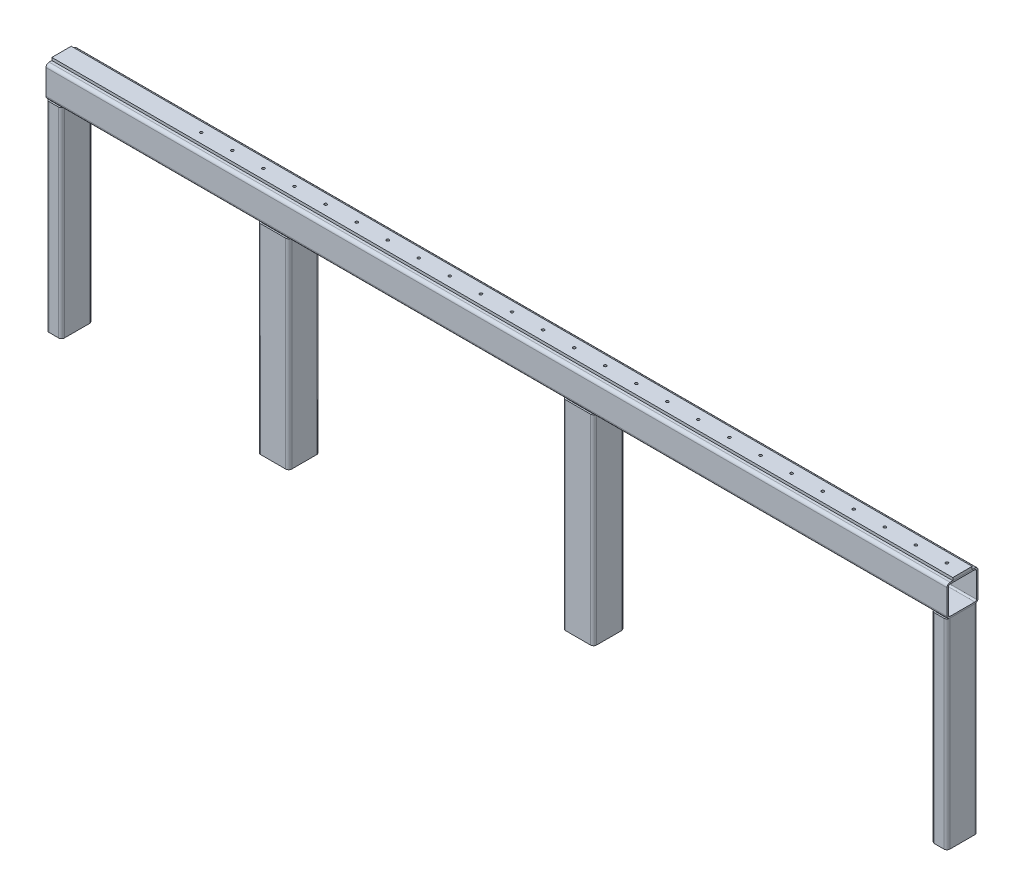
SolidWorks part; units mm, degrees
material "Q235"
ref_plane "Front Plane" through (0, 0, 0) normal (0, 0, 1) x (1, 0, 0)
ref_plane "Top Plane" through (0, 0, 0) normal (0, 1, 0) x (1, 0, 0)
ref_plane "Right Plane" through (0, 0, 0) normal (1, 0, 0) x (0, 0, -1)
sketch "草图1" plane through (0, 0, 0) normal (0, 0, 1) x (1, 0, 0)
  line L0 (0, 0) -> (0, 515)
  line L1 (0, 515) -> (2280, 515)
  line L2 (2280, 515) -> (2280, 0)
  line L3 (565, 515) -> (565, 0)
  line L4 (1350, 515) -> (1350, 0)
  dimension "D1" = 2280
  dimension "D2" = 515
  dimension "D3" = 565
  dimension "D4" = 785
other "GB/6728-1986 rect hollow section 080 X 40 X 4(1)"
ref_plane "Plane2" through (0, 0, 0) normal (0, 1, 0) x (-1, 0, 0)
sketch "Sketch11" plane through (0, 0, 0) normal (0, 1, 0) x (-1, 0, 0)
  line L0 (-12, -36) -> (12, -36)
  line L1 (-16, -32) -> (-16, 32)
  line L2 (12, 36) -> (-12, 36)
  line L3 (16, 32) -> (16, -32)
  line L4 (-12, -40) -> (12, -40)
  line L5 (-20, -32) -> (-20, 32)
  line L6 (12, 40) -> (-12, 40)
  line L7 (20, 32) -> (20, -32)
  arc A0 (20, 32) -> (12, 40) centre (12, 32) ccw
  arc A1 (12, -40) -> (20, -32) centre (12, -32) ccw
  arc A2 (-20, -32) -> (-12, -40) centre (-12, -32) ccw
  arc A3 (-12, 40) -> (-20, 32) centre (-12, 32) ccw
  arc A4 (-12, 36) -> (-16, 32) centre (-12, 32) ccw
  arc A5 (16, 32) -> (12, 36) centre (12, 32) ccw
  arc A6 (12, -36) -> (16, -32) centre (12, -32) ccw
  arc A7 (-16, -32) -> (-12, -36) centre (-12, -32) ccw
  point P0 (0, 40)
  point P1 (20, 0)
  point P2 (0, -40)
  point P3 (-20, 0)
  point P4 (-20, 40)
  point P5 (20, 40)
  point P6 (20, -40)
  point P7 (-20, -40)
  point P8 (0, 0)
  point P33 (0, 0)
  dimension "D1" = 8
  dimension "Thickness" = 4
  dimension "V_leg" = 80
  dimension "H_leg" = 40
other "GB/6728-1986 square hollow section 080 X 80 X 4(1)"
ref_plane "Plane1" through (0, 555, 0) normal (1, 0, 0) x (0, 1, 0)
sketch "Sketch1" plane through (0, 555, 0) normal (1, 0, 0) x (0, 1, 0)
  line L0 (-32, -36) -> (32, -36)
  line L1 (-36, -32) -> (-36, 32)
  line L2 (32, 36) -> (-32, 36)
  line L3 (36, 32) -> (36, -32)
  line L4 (-32, -40) -> (32, -40)
  line L5 (-40, -32) -> (-40, 32)
  line L6 (32, 40) -> (-32, 40)
  line L7 (40, 32) -> (40, -32)
  arc A0 (40, 32) -> (32, 40) centre (32, 32) ccw
  arc A1 (32, -40) -> (40, -32) centre (32, -32) ccw
  arc A2 (-40, -32) -> (-32, -40) centre (-32, -32) ccw
  arc A3 (-32, 40) -> (-40, 32) centre (-32, 32) ccw
  arc A4 (-32, 36) -> (-36, 32) centre (-32, 32) ccw
  arc A5 (36, 32) -> (32, 36) centre (32, 32) ccw
  arc A6 (32, -36) -> (36, -32) centre (32, -32) ccw
  arc A7 (-36, -32) -> (-32, -36) centre (-32, -32) ccw
  point P0 (-40, 0)
  point P1 (40, 0)
  point P2 (0, 40)
  point P3 (0, -40)
  point P4 (0, 0)
  point P5 (-40, -40)
  point P6 (40, -40)
  point P7 (40, 40)
  point P8 (-40, 40)
  point P33 (0, 0)
  dimension "D1" = 8
  dimension "Thickness" = 4
  dimension "V_leg" = 80
other "Trim/extend1"
other "Trim/extend2"
sketch "Sketch2" plane through (0, 595, 0) normal (0, 1, 0) x (1, 0, 0)
  line L0 (-20, -32) -> (-20, 32) construction
  line L1 (-20, 25) -> (2300, 25)
  line L2 (-20, 25) -> (-20, -25)
  line L3 (-20, -25) -> (2300, -25)
  line L4 (2300, 25) -> (2300, -25)
  line L5 (2300, 32) -> (2300, -32) construction
  line L6 (2300, -40) -> (-20, -40) construction
  dimension "D1" = 50
  dimension "D2" = 15
extrude "Boss-Extrude1" add sketch "Sketch2" along normal blind 10 separate body
sketch "Sketch4" plane through (0, 605, 0) normal (0, 1, 0) x (1, 0, 0)
  line L0 (-20, 25) -> (-20, -25) construction
  line L1 (-20, 25) -> (2300, 25)
  line L2 (-20, 25) -> (-20, -25)
  line L3 (-20, -25) -> (2300, -25)
  line L4 (2300, 25) -> (2300, -25)
  line L5 (2300, -25) -> (2300, 25) construction
  line L6 (2300, 0) -> (2032.1771, 0) construction
  dimension "D1" = 50
extrude "Cut-Extrude1" cut sketch "Sketch4" against normal blind 3
hole_wizard "M8 Tapped Hole1" positions "Sketch5" profile "Sketch6" tap size "M8" standard "GB"
sketch "Sketch5" plane through (0, 602, 0) normal (0, 1, 0) x (1, 0, 0)
  line L0 (2300, 0) -> (2260, 0) construction
  line L1 (2300, -25) -> (2300, 25) construction
  point P0 (2260, 0)
  dimension "D1" = 40
sketch "Sketch6" plane through (2260, 602, 0) normal (1, 0, 0) x (0, 0, 1)
  line L0 (0, 0) -> (0, 21.7929)
  line L1 (0, 21.7929) -> (3.4, 19.75)
  line L2 (3.4, 19.75) -> (3.4, 0)
  line L5 (3.4, 0) -> (0, 0)
  line L10 (0, 21.7929) -> (-3.4, 19.75) construction
  line L11 (0, -6.35) -> (0, 107.95) construction
  dimension "螺纹孔钻头直径" = 6.8
  dimension "螺纹孔钻头深度" = 19.75
  dimension "导头角度" = 118
cosmetic thread "Hole thread1"
pattern_linear "LPattern1" count 25 spacing 80 along (-1, 0, 0) of "M8 Tapped Hole1"
other "Square tube 80 X 80 X 4.0(1)"
ref_plane "Plane3" through (565, 515, 0) normal (0, -1, 0) x (1, 0, 0)
sketch "Sketch12" plane through (565, 515, 0) normal (0, -1, 0) x (1, 0, 0)
  line L0 (-32, -36) -> (32, -36)
  line L1 (-36, -32) -> (-36, 32)
  line L2 (32, 36) -> (-32, 36)
  line L3 (36, 32) -> (36, -32)
  line L4 (-32, -40) -> (32, -40)
  line L5 (-40, -32) -> (-40, 32)
  line L6 (32, 40) -> (-32, 40)
  line L7 (40, 32) -> (40, -32)
  line L8 (-40, 0) -> (-36, 0) construction
  line L9 (-36, 0) -> (36, 0) construction
  line L10 (36, 0) -> (40, 0) construction
  line L12 (0, 40) -> (0, 36) construction
  line L13 (0, 36) -> (0, -36) construction
  line L14 (0, -36) -> (0, -40) construction
  arc A0 (40, 32) -> (32, 40) centre (32, 32) ccw
  arc A1 (32, -40) -> (40, -32) centre (32, -32) ccw
  arc A2 (-40, -32) -> (-32, -40) centre (-32, -32) ccw
  arc A3 (-32, 40) -> (-40, 32) centre (-32, 32) ccw
  arc A4 (-32, 36) -> (-36, 32) centre (-32, 32) ccw
  arc A5 (36, 32) -> (32, 36) centre (32, 32) ccw
  arc A6 (32, -36) -> (36, -32) centre (32, -32) ccw
  arc A7 (-36, -32) -> (-32, -36) centre (-32, -32) ccw
  point P2 (-40, 40)
  point P33 (-40, -40)
  point P34 (40, -40)
  point P36 (40, 40)
  point P37 (0, 0)
  dimension "D1" = 8
  dimension "Thickness" = 4
  dimension "V_leg" = 80
  dimension "H_leg" = 80
